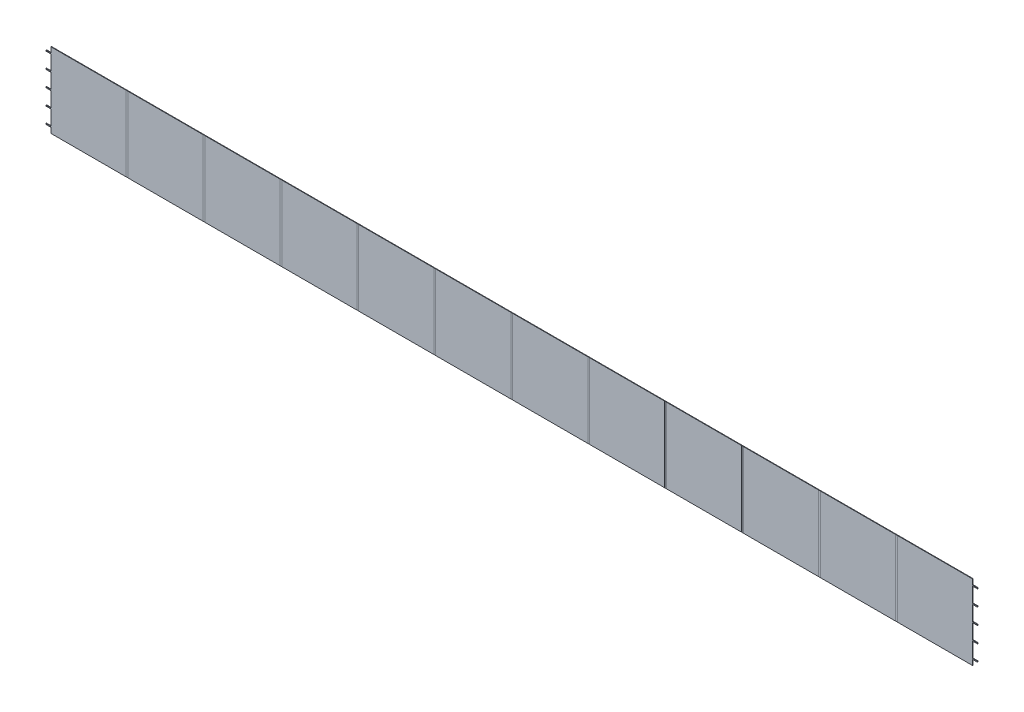
from build123d import *

# Parameters (mm, degrees)
SKETCH_1_W      = 1916
SKETCH_1_H      = 156
EXTRUDE_1_DEPTH = 1
SKETCH_2_W      = 156
SKETCH_2_H      = 156
EXTRUDE_2_DEPTH = 0.1
SKETCH_3_W      = 20
SKETCH_3_H      = 2
EXTRUDE_3_DEPTH = 1.1


with BuildPart() as part:
    # 草图1 → 凸台-拉伸1 (new body)
    with BuildSketch(Plane.XY):
        with Locations((958, -78)):
            Rectangle(SKETCH_1_W, SKETCH_1_H)
    extrude(amount=EXTRUDE_1_DEPTH)

    # 草图2 → 凸台-拉伸2 (add)
    with BuildSketch(Plane.XY.offset(1)):
        with Locations((78, -78)):
            Rectangle(SKETCH_2_W, SKETCH_2_H)
        with Locations((238, -78)):
            Rectangle(SKETCH_2_W, SKETCH_2_H)
        with Locations((398, -78)):
            Rectangle(SKETCH_2_W, SKETCH_2_H)
        with Locations((558, -78)):
            Rectangle(SKETCH_2_W, SKETCH_2_H)
        with Locations((718, -78)):
            Rectangle(SKETCH_2_W, SKETCH_2_H)
        with Locations((878, -78)):
            Rectangle(SKETCH_2_W, SKETCH_2_H)
        with Locations((1038, -78)):
            Rectangle(SKETCH_2_W, SKETCH_2_H)
        with Locations((1198, -78)):
            Rectangle(SKETCH_2_W, SKETCH_2_H)
        with Locations((1358, -78)):
            Rectangle(SKETCH_2_W, SKETCH_2_H)
        with Locations((1518, -78)):
            Rectangle(SKETCH_2_W, SKETCH_2_H)
        with Locations((1678, -78)):
            Rectangle(SKETCH_2_W, SKETCH_2_H)
        with Locations((1838, -78)):
            Rectangle(SKETCH_2_W, SKETCH_2_H)
    extrude(amount=EXTRUDE_2_DEPTH)

    # 草图3 → 凸台-拉伸3 (add)
    with BuildSketch(Plane.XY.offset(1.1)):
        with Locations((0, -12)):
            Rectangle(SKETCH_3_W, SKETCH_3_H)
        with Locations((0, -45)):
            Rectangle(SKETCH_3_W, SKETCH_3_H)
        with Locations((0, -78)):
            Rectangle(SKETCH_3_W, SKETCH_3_H)
        with Locations((0, -111)):
            Rectangle(SKETCH_3_W, SKETCH_3_H)
        with Locations((0, -144)):
            Rectangle(SKETCH_3_W, SKETCH_3_H)
    extrude_3 = extrude(amount=-EXTRUDE_3_DEPTH)

    # 镜向1: 凸台-拉伸3 across plane
    add(extrude_3.mirror(Plane.ZY.offset(-958)))


solid = part.part
